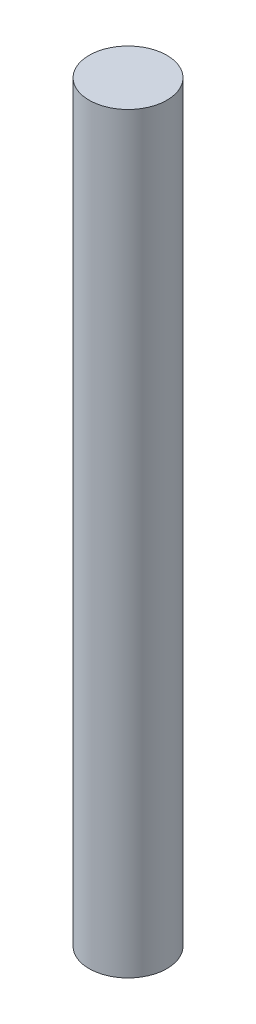
from build123d import *

# Parameters (mm, degrees)
SKETCH_1_R      = 3
SKETCH_1_R_2    = 1.5
EXTRUDE_1_DEPTH = 58


with BuildPart() as part:
    # 草图1 → 凸台-拉伸1 (new body)
    # profile 1 of 2: a face of its own
    with BuildSketch(Plane(origin=(0, 0, 0), x_dir=(1, 0, 0), z_dir=(0, 1, 0))):
        with Locations(Location((0, 0, 0), (0, 0, 90))):
            Circle(SKETCH_1_R)
        Circle(SKETCH_1_R_2, mode=Mode.SUBTRACT)
    # profile 2 of 2: a face of its own
    with BuildSketch(Plane(origin=(0, 0, 0), x_dir=(1, 0, 0), z_dir=(0, 1, 0))):
        Circle(SKETCH_1_R_2)
    extrude(amount=EXTRUDE_1_DEPTH)


solid = part.part
